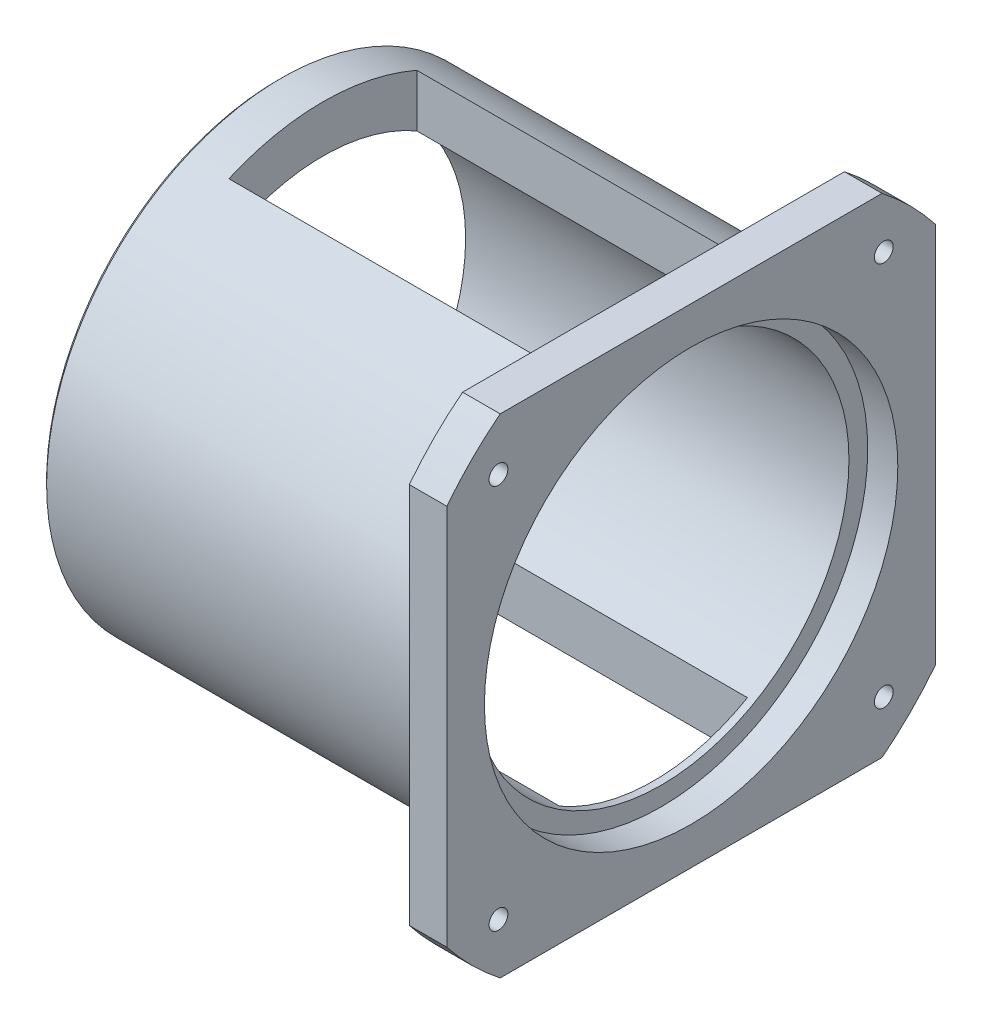
SolidWorks part; units mm, degrees
ref_plane "前视基准面" through (0, 0, 0) normal (0, 0, 1) x (1, 0, 0)
ref_plane "上视基准面" through (0, 0, 0) normal (0, 1, 0) x (1, 0, 0)
ref_plane "右视基准面" through (0, 0, 0) normal (1, 0, 0) x (0, 0, -1)
sketch "草图1" plane through (0, 0, 0) normal (1, 0, 0) x (0, 0, -1)
  circle A0 centre (0, 0) radius 62.5
  dimension "D1" = 125
extrude "凸台-拉伸1" add sketch "草图1" along normal blind 100
sketch "草图2" plane through (100, 0, 0) normal (1, 0, 0) x (0, 0, -1)
  circle A0 centre (0, 0) radius 82.5
  dimension "D1" = 165
extrude "凸台-拉伸2" add sketch "草图2" along normal blind 10
sketch "草图3" plane through (110, 0, 0) normal (1, 0, 0) x (0, 0, -1)
  line L0 (0, 132.3949) -> (0, 0) construction
  line L1 (-65, 65) -> (65, 65)
  line L2 (-65, 65) -> (-65, -65)
  line L3 (-65, -65) -> (65, -65)
  line L4 (65, 65) -> (65, -65)
  line L5 (0, 0) -> (118.7422, 0) construction
  dimension "D1" = 130
extrude "切除-拉伸1" cut sketch "草图3" against normal through all flip side to cut
sketch "草图4" plane through (110, 0, 0) normal (1, 0, 0) x (0, 0, -1)
  circle A0 centre (0, 0) radius 55
  dimension "D1" = 110
extrude "切除-拉伸2" cut sketch "草图4" against normal blind 8
hole_wizard "M6 螺纹孔1" positions "草图5" profile "草图6" tap size "M6" standard "GB"
sketch "草图5" plane through (110, 0, 0) normal (1, 0, 0) x (0, 0, -1)
  line L0 (0, 0) -> (0, 62.713) construction
  line L2 (0, 0) -> (-51.2652, 51.2652) construction
  point P0 (-51.2652, 51.2652)
  dimension "D1" = 45
  dimension "D2" = 72.5
sketch "草图6" plane through (110, 51.2652, 51.2652) normal (0, 1, 0) x (0, 0, -1)
  line L0 (0, 0) -> (0, 16.5022)
  line L1 (0, 16.5022) -> (2.5, 15)
  line L2 (2.5, 15) -> (2.5, 0)
  line L5 (2.5, 0) -> (0, 0)
  line L10 (0, 16.5022) -> (-2.5, 15) construction
  line L11 (0, -6.35) -> (0, 107.95) construction
  dimension "螺纹孔钻头直径" = 5
  dimension "螺纹孔钻头深度" = 15
  dimension "导头角度" = 118
cosmetic thread "孔螺蚊线1" parameters "D1"=10, "D2"=6
pattern_circular "阵列(圆周)1" count 4 over 360 about axis through (0, 0, 0) along (1, 0, 0) of "M6 螺纹孔1"
sketch "草图7" plane through (102, 0, 0) normal (1, 0, 0) x (0, 0, -1)
  circle A0 centre (0, 0) radius 50
  dimension "D1" = 100
extrude "切除-拉伸3" cut sketch "草图7" against normal through all
sketch "草图8" plane through (0, 0, 0) normal (0, 1, 0) x (1, 0, 0)
  line L0 (0, 0) -> (80.8943, 0) construction
  line L1 (12, 25) -> (100, 25)
  line L2 (12, 25) -> (12, -25)
  line L3 (12, -25) -> (100, -25)
  line L4 (100, 25) -> (100, -25)
  line L5 (100, 50.806) -> (100, -50.806) construction
  line L6 (0, 62.5) -> (0, -62.5) construction
  dimension "D1" = 50
  dimension "D2" = 12
extrude "切除-拉伸4" cut sketch "草图8" against normal through all both and the other way through all
hole_wizard "M8 螺纹孔1" positions "草图9" profile "草图10" tap size "M8" standard "GB"
sketch "草图9" plane through (0, 0, 0) normal (-1, 0, 0) x (0, 0, 1)
  line L0 (-39.598, 39.598) -> (0, 0) construction
  line L1 (0, 0) -> (0, 41.5769) construction
  point P0 (-39.598, 39.598)
  dimension "D1" = 45
  dimension "D2" = 56
sketch "草图10" plane through (0, 39.598, -39.598) normal (0, 1, 0) x (0, 0, 1)
  line L0 (0, 0) -> (0, 21.7929)
  line L1 (0, 21.7929) -> (3.4, 19.75)
  line L2 (3.4, 19.75) -> (3.4, 0)
  line L5 (3.4, 0) -> (0, 0)
  line L10 (0, 21.7929) -> (-3.4, 19.75) construction
  line L11 (0, -6.35) -> (0, 107.95) construction
  dimension "螺纹孔钻头直径" = 6.8
  dimension "螺纹孔钻头深度" = 19.75
  dimension "导头角度" = 118
cosmetic thread "孔螺蚊线2" parameters "D1"=16, "D2"=8
pattern_circular "阵列(圆周)2" count 4 over 360 about axis through (0, 0, 0) along (1, 0, 0) of "M8 螺纹孔1"
chamfer "倒角1" distance 1 angle 45 1 edges at (0, 0, -62.5)
